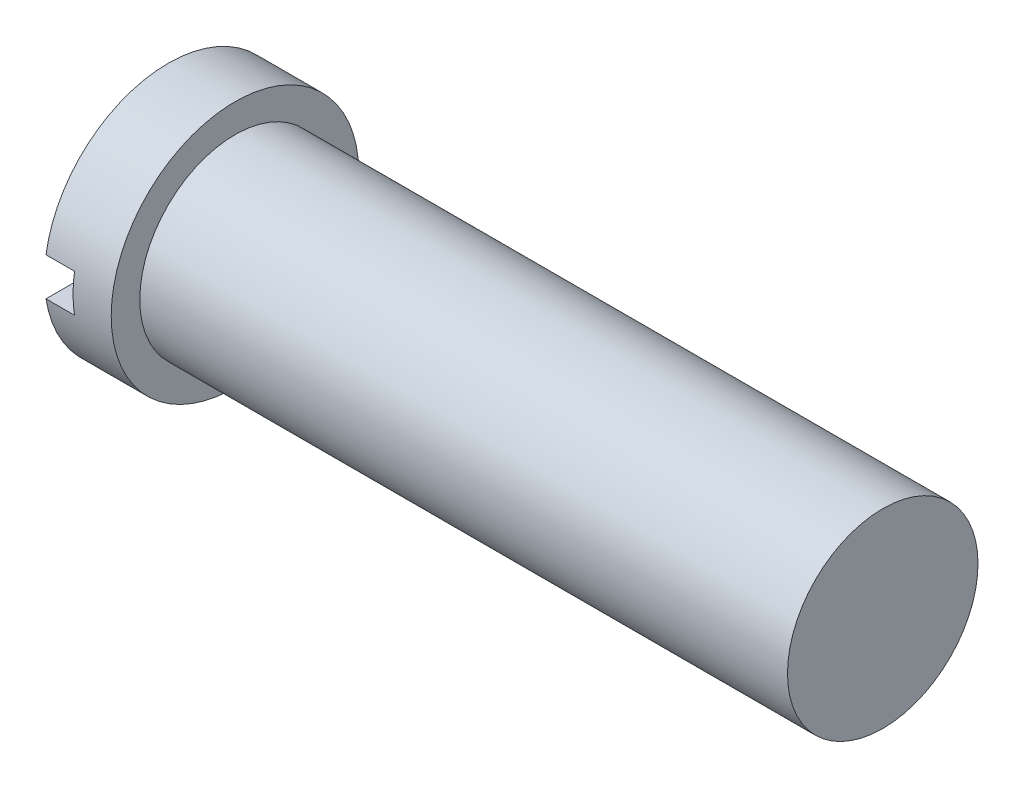
SolidWorks part; units mm, degrees
ref_plane "前视基准面" through (0, 0, 0) normal (0, 0, 1) x (1, 0, 0)
ref_plane "上视基准面" through (0, 0, 0) normal (0, 1, 0) x (1, 0, 0)
ref_plane "右视基准面" through (0, 0, 0) normal (1, 0, 0) x (0, 0, -1)
sketch "草图1" plane through (0, 0, 0) normal (0, 0, 1) x (1, 0, 0)
  line L0 (-19.4211, 0) -> (53.8682, 0) construction
  line L1 (0, 0) -> (0, 6.5)
  line L2 (0, 6.5) -> (3.5, 6.5)
  line L3 (3.5, 6.5) -> (3.5, 5)
  line L4 (3.5, 5) -> (47.5, 5)
  line L5 (47.5, 5) -> (47.5, 0)
  line L6 (0, 0) -> (47.5, 0)
  dimension "D1" = 6.5
  dimension "D2" = 5
  dimension "D3" = 3.5
  dimension "D4" = 44
revolve "旋转1" add sketch "草图1" angle 360 about L0
cosmetic thread "装饰螺纹线2" parameters "D1"=4, "D2"=8.917
chamfer "倒角2" distance 1 angle 45 1 edges at (47.5, 0, 5)
sketch "草图2" plane through (0, 0, 0) normal (0, 0, 1) x (1, 0, 0)
  line L0 (0, 0) -> (3.036, 0) construction
  line L1 (1.5, -1) -> (0, -1)
  line L2 (1.5, -1) -> (1.5, 1)
  line L3 (0, -1) -> (0, 1)
  line L4 (1.5, 1) -> (0, 1)
  line L5 (1.5, -1) -> (0, 1) construction
  line L6 (0, -1) -> (1.5, 1) construction
  line L7 (0, 6.5) -> (0, -6.5) construction
  point P4 (0.75, 0)
  dimension "D1" = 1.5
  dimension "D2" = 2
extrude "切除-拉伸1" cut sketch "草图2" against normal through all and the other way through all
sketch "草图3" plane through (47.5, 0, 0) normal (1, 0, 0) x (0, 0, -1)
  circle A0 centre (0, 0) radius 5.5
  dimension "D1" = 11
extrude "切除-拉伸2" cut sketch "草图3" against normal blind 10
